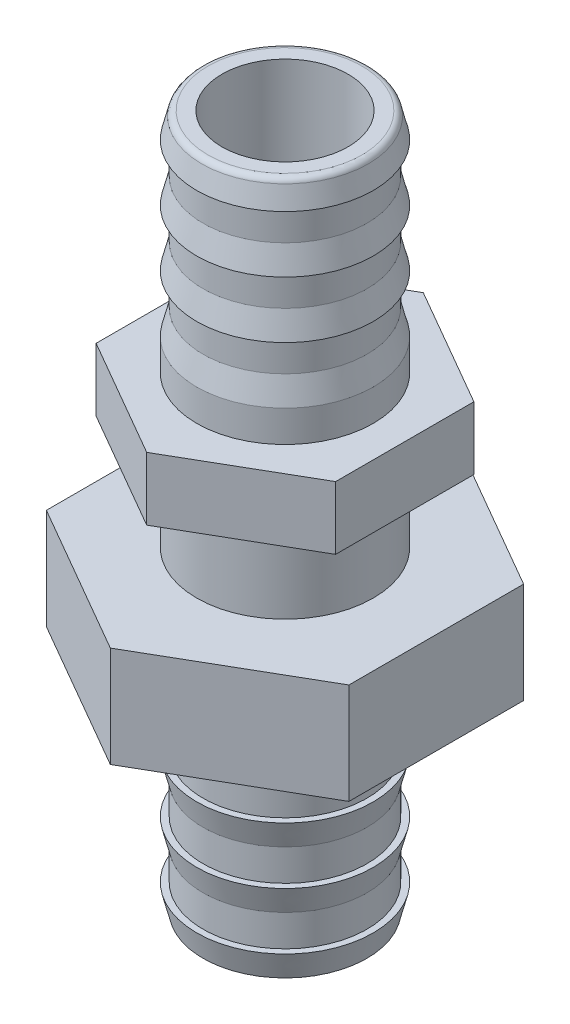
from build123d import *

# Parameters (mm, degrees)
SKETCH2_R           = 7
BOSS_EXTRUDE1_DEPTH = 18
BOSS_EXTRUDE2_DEPTH = 5
BOSS_EXTRUDE3_START = 32
SKETCH6_R           = 7
BOSS_EXTRUDE3_DEPTH = 32
SKETCH4_R           = 5
CUT_EXTRUDE1_DEPTH  = 57.88218819
FILLET1_R           = 0.5
SKETCH8_R           = 7
BOSS_EXTRUDE4_DEPTH = 8


with BuildPart() as part:
    # Sketch2 → Boss-Extrude1 (new body)
    with BuildSketch(Plane(origin=(0, 0, 0), x_dir=(1, 0, 0), z_dir=(0, 1, 0))):
        with Locations(Location((0, 0, 0), (0, 0, 270))):
            Circle(SKETCH2_R)
    extrude(amount=BOSS_EXTRUDE1_DEPTH)

    # Sketch5 → Boss-Extrude2 (add)
    with BuildSketch(Plane.XZ):
        Polygon((9.5, -5.484827557), (9.5, 5.484827557), (0, 10.969655115), (-9.5, 5.484827557), (-9.5, -5.484827557), (0, -10.969655115), align=None)
    extrude(amount=BOSS_EXTRUDE2_DEPTH)

    # Sketch6 → Boss-Extrude3 (add)
    with BuildSketch(Plane.XZ.offset(5).offset(BOSS_EXTRUDE3_START)):
        with Locations(Location((0, 0, 0), (0, 0, 90))):
            Circle(SKETCH6_R)
    extrude(amount=-BOSS_EXTRUDE3_DEPTH)

    # Sketch4 → Cut-Extrude1 (cut, through all)
    with BuildSketch(Plane(origin=(0, 18, 0), x_dir=(1, 0, 0), z_dir=(0, 1, 0))):
        with Locations(Location((0, 0, 0), (0, 0, 270))):
            Circle(SKETCH4_R)
    extrude(amount=-CUT_EXTRUDE1_DEPTH, mode=Mode.SUBTRACT)

    # Sketch3 → Cut-Revolve1 (revolve, cut)
    with BuildSketch(Plane.XY, mode=Mode.PRIVATE) as cut_revolve1_sk:
        Polygon((6.5, 18), (7, 16), (6.5, 16), (6.5, 13.5), (7, 11.5), (6.5, 11.5), (6.5, 9), (7, 7), (6.5, 7), (6.5, 4.5), (7, 2.5), (7, 18), align=None)
        Polygon((6.5, -23.5), (7, -21.5), (7, -37), (6.5, -37), (7, -35), (6.5, -35), (6.5, -32.5), (7, -30.5), (6.5, -30.5), (6.5, -28), (7, -26), (6.5, -26), align=None)
    revolve(cut_revolve1_sk.sketch.rotate(Axis((0, 0, 0), (0, 1, 0)), 90), axis=Axis((0, 0, 0), (0, 1, 0)), mode=Mode.SUBTRACT)

    # Fillet1
    fillet1_edges = [part.edges().sort_by_distance(p)[0] for p in [
        (0, 18, 6.5),
    ]]
    fillet(fillet1_edges, radius=FILLET1_R)


with BuildPart() as body_2:
    # Sketch8 → Boss-Extrude4 (new body)
    with BuildSketch(Plane(origin=(0, -12, 0), x_dir=(-1, 0, 0), z_dir=(0, -1, 0))):
        Polygon((0, 13.856406461), (-12, 6.92820323), (-12, -6.92820323), (0, -13.856406461), (12, -6.92820323), (12, 6.92820323), align=None)
        with Locations(Location((0, 0, 0), (0, 0, 90))):
            Circle(SKETCH8_R, mode=Mode.SUBTRACT)
    extrude(amount=BOSS_EXTRUDE4_DEPTH)


solid = Compound([part.part, body_2.part])
